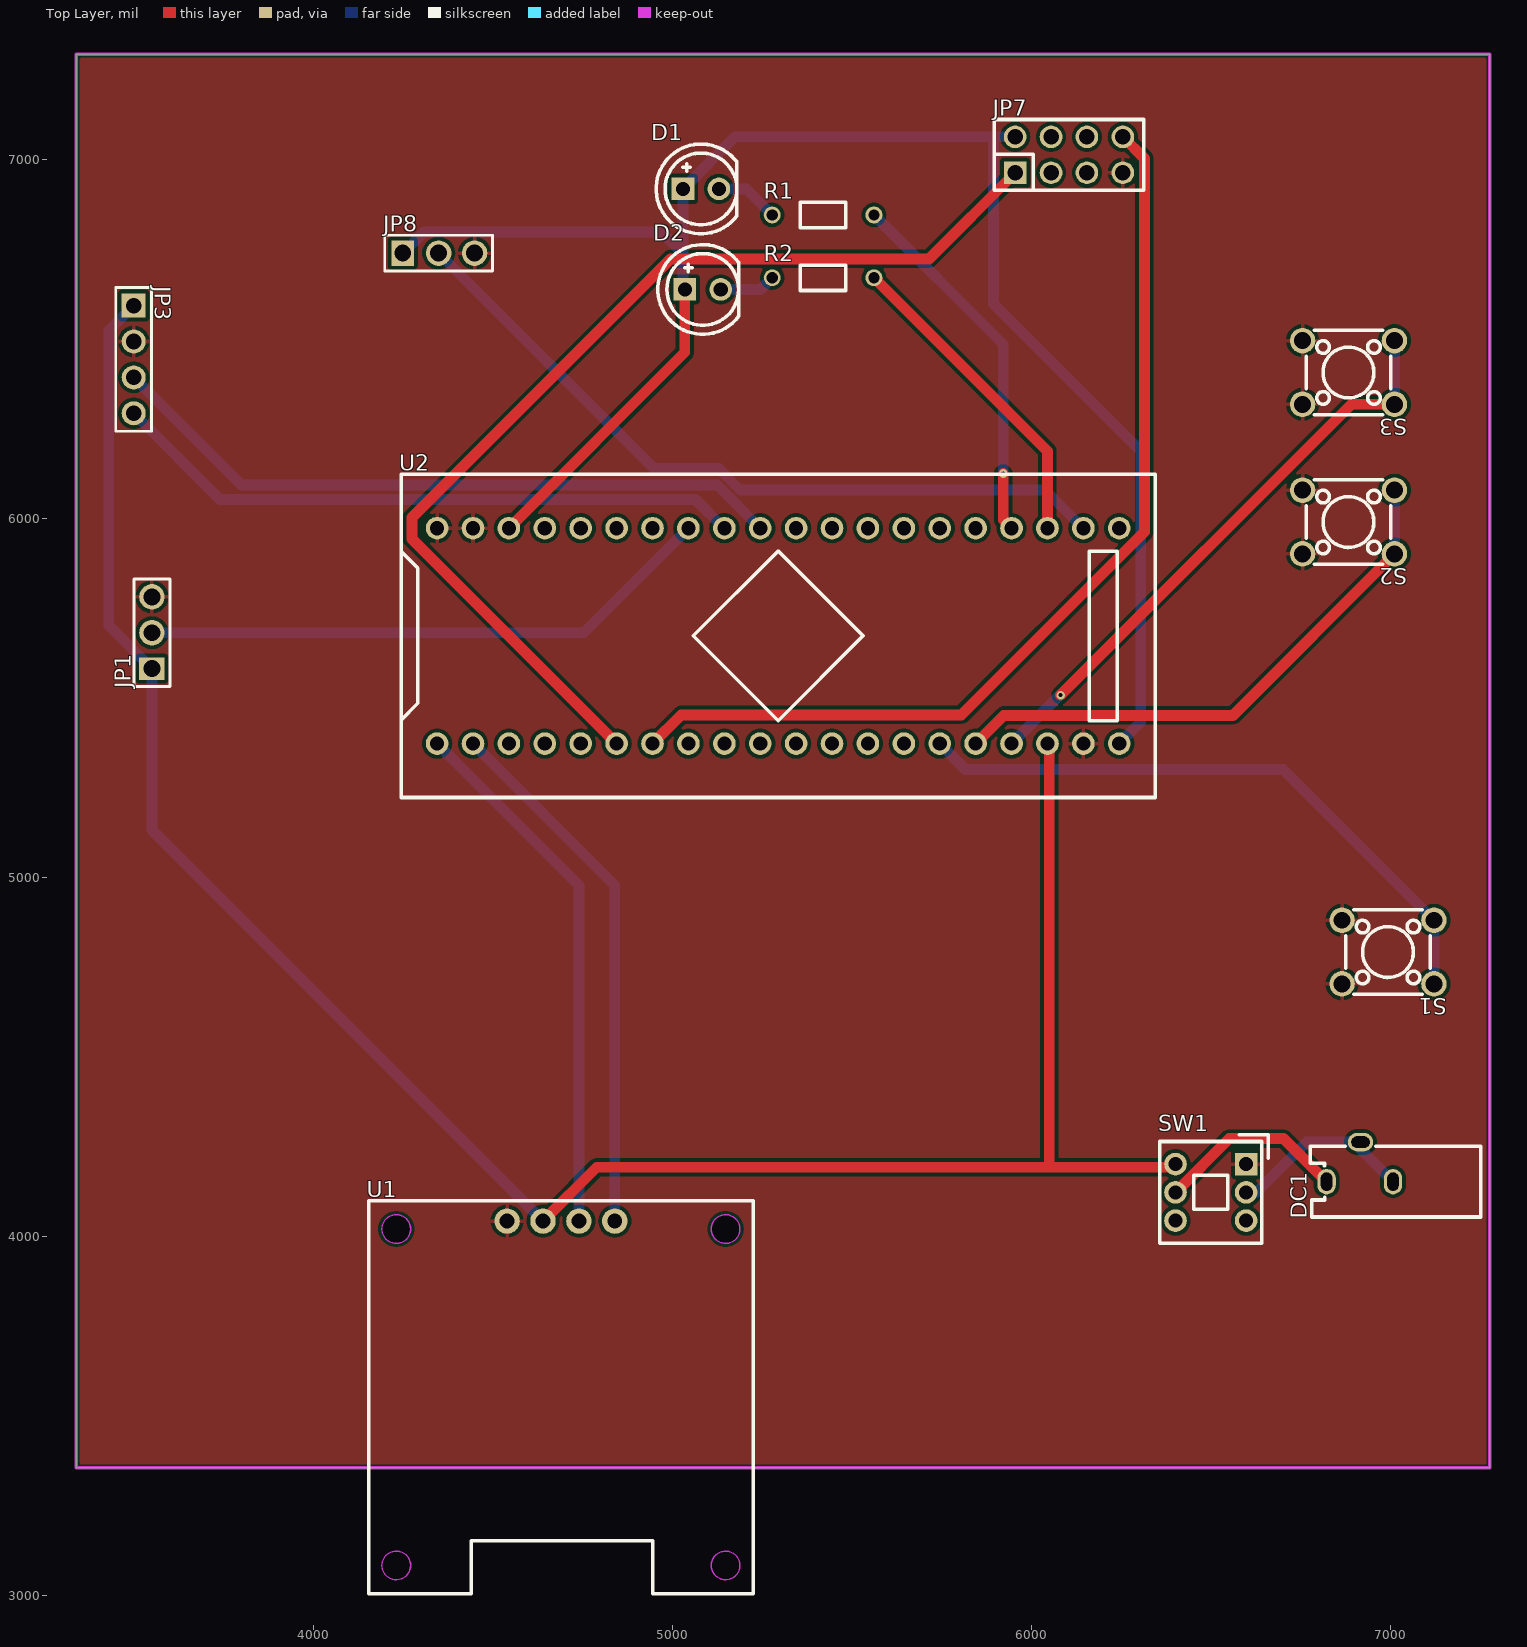
[diagram p0: Top Layer view]
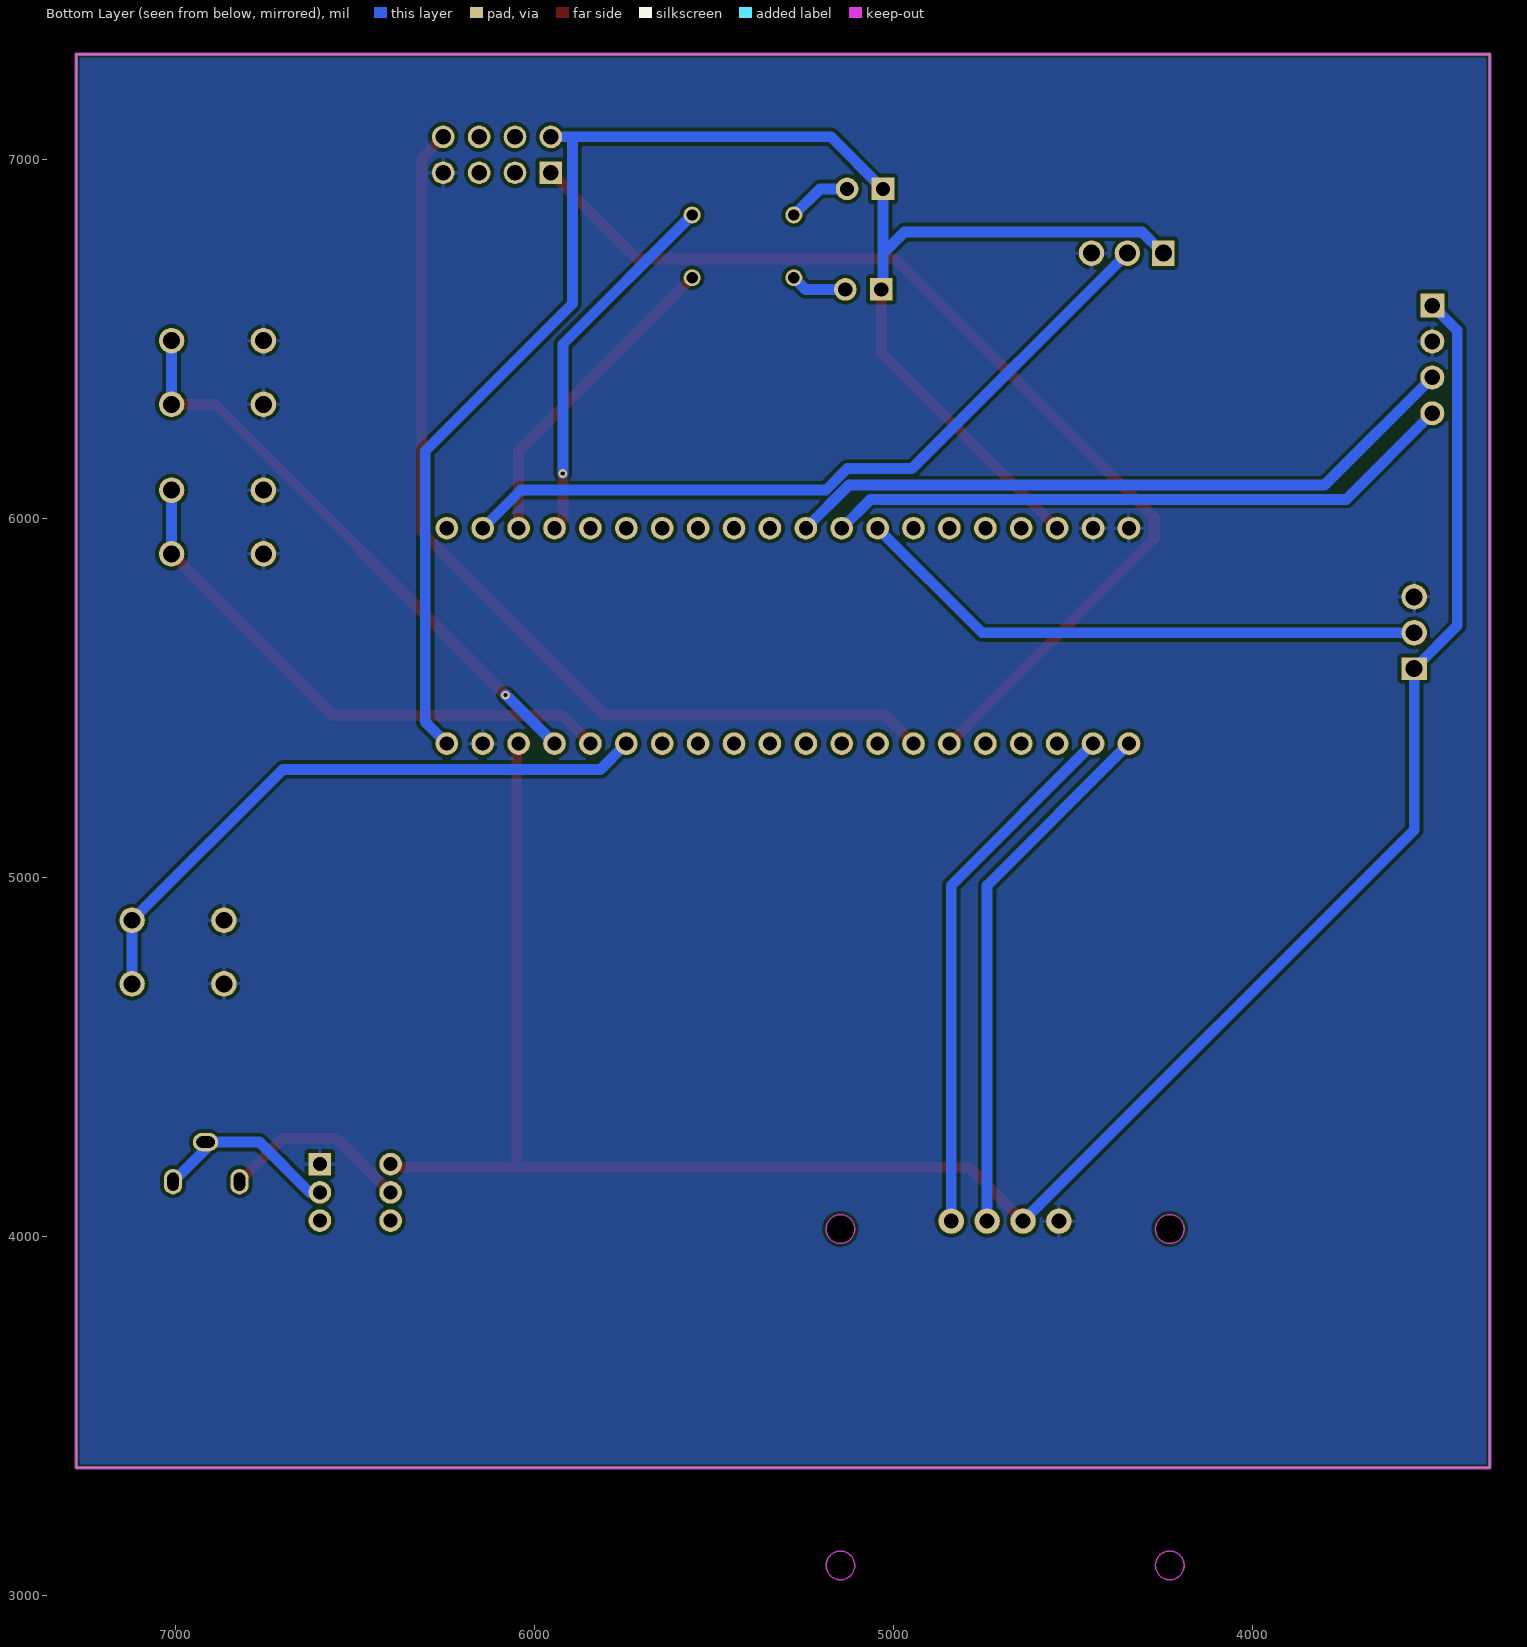
[diagram p1: Bottom Layer view, seen from below]
# Altium PCB MISC51894.pcbdoc
Units mil, origin at the board's own origin, x right, y up, seen from the top; angles counter-clockwise.
Board outline 3937.01 x 3937.01 mil, 2 copper layers (Top Layer, Bottom Layer), stack 62.206 mil thick; 15 components, 45 nets, 91 pads, 2 vias.

## Layer stack, top to bottom
Top Solder Mask Layer: solder mask 0.394, Dk 3.3
Top Layer: signal copper 1.379
Dielectric1: surface 59.449, FR4, Dk 4.5
Bottom Layer: signal copper 1.378
Bottom Solder Mask Layer: solder mask 0.394, Dk 3.3

## Board outline
3340,7292.79 3340,3355.79 7277.01,3355.79 7277.01,7292.79

## Design rules (kind name [scope] priority, off if disabled: settings)
BoardOutlineClearance copperThickness2oz_1 [All] p2 off: genericclearance=7.99 ignorepadtopadclearanceinfootprint=FALSE except(0: Arc-SplitContinuation Track-SplitContinuation SMDPad-SplitContinuation THPad-SplitContinuation Via-SplitContinuation Fill-SplitContinuation Region-SplitContinuation Poly-SplitContinuation Text-SplitContinuation Hole-SplitContinuation; 5.98: Arc-CutoutEdge SMDPad-CutoutEdge THPad-CutoutEdge Via-CutoutEdge Fill-CutoutEdge Region-CutoutEdge Text-CutoutEdge; 6.93: Hole-OutlineEdge Hole-CutoutEdge; 10: Poly-OutlineEdge Poly-CutoutEdge; 11.81: Arc-OutlineEdge Track-OutlineEdge SMDPad-OutlineEdge THPad-OutlineEdge Via-OutlineEdge Fill-OutlineEdge Region-OutlineEdge Text-OutlineEdge Track-CutoutEdge)
BoardOutlineClearance copperThickness1oz_1 [All] p4: genericclearance=4.02 ignorepadtopadclearanceinfootprint=FALSE except(0: Arc-SplitContinuation Track-SplitContinuation SMDPad-SplitContinuation THPad-SplitContinuation Via-SplitContinuation Fill-SplitContinuation Region-SplitContinuation Poly-SplitContinuation Text-SplitContinuation Hole-SplitContinuation; 6: SMDPad-CutoutEdge THPad-CutoutEdge Via-CutoutEdge Fill-CutoutEdge Region-CutoutEdge Text-CutoutEdge; 6.93: Hole-OutlineEdge Hole-CutoutEdge; 10: Poly-OutlineEdge Poly-CutoutEdge; 11.8: Arc-OutlineEdge Track-OutlineEdge SMDPad-OutlineEdge THPad-OutlineEdge Via-OutlineEdge Fill-OutlineEdge Region-OutlineEdge Text-OutlineEdge; 11.81: Arc-CutoutEdge Track-CutoutEdge)
Clearance copperThickness2oz [All] p1 off: gap=7.99 ignorepadtopadclearanceinfootprint=FALSE except(5.98: SMDPad-Track SMDPad-SMDPad THPad-Track SMDPad-THPad THPad-THPad Track-Via SMDPad-Via THPad-Via Via-Via Fill-Track Region-Track Fill-SMDPad Region-SMDPad Fill-THPad Region-THPad Fill-Via Region-Via Fill-Fill Fill-Region Region-Region Arc-Track Arc-SMDPad Arc-THPad Arc-Via Fill-Arc Region-Arc Arc-Arc Text-Track SMDPad-Text Text-THPad Text-Via Fill-Text Region-Text Arc-Text Text-Text; 6.93: Hole-Track Hole-SMDPad Hole-THPad Hole-Via Fill-Hole Region-Hole Hole-Arc Hole-Text; 10: Poly-Track Poly-SMDPad Poly-THPad Poly-Via Poly-Fill Poly-Region Poly-Poly Poly-Arc Poly-Text Poly-Hole)
Clearance copperThickness1oz [All] p3: gap=4.02 ignorepadtopadclearanceinfootprint=FALSE except(5.98: SMDPad-Track SMDPad-SMDPad THPad-Track SMDPad-THPad THPad-THPad Track-Via SMDPad-Via THPad-Via Via-Via Fill-Track Region-Track Fill-SMDPad Region-SMDPad Fill-THPad Region-THPad Fill-Via Region-Via Fill-Fill Fill-Region Region-Region; 6: Arc-Track Arc-SMDPad Arc-THPad Arc-Via Fill-Arc Region-Arc Arc-Arc Text-Track SMDPad-Text Text-THPad Text-Via Fill-Text Region-Text Arc-Text Text-Text; 6.93: Hole-Track Hole-SMDPad Hole-THPad Hole-Via Fill-Hole Region-Hole Hole-Arc Hole-Text; 10: Poly-Track Poly-SMDPad Poly-THPad Poly-Via Poly-Fill Poly-Region Poly-Poly Poly-Arc Poly-Text Poly-Hole)
Creepage creepage [All] p1: checkdistance=0 ignoreinternallayers=TRUE applytopolygonpour=TRUE
DiffPairsRouting differentialPair [All] p1: maxlimit=6 minlimit=6 mostfreqgap=6 toplayer_minwidth=5 toplayer_prefwidth=10 toplayer_maxwidth=100 toplayer_mingap=6 toplayer_prefgap=6 toplayer_maxgap=6 bottomlayer_minwidth=5 bottomlayer_prefwidth=10 bottomlayer_maxwidth=100 bottomlayer_mingap=6 bottomlayer_prefgap=6 bottomlayer_maxgap=6 maxuncoupledlength=10
HoleToHoleClearance otherClearance [All] p1: gap=11.81 allowstackedmicrovias=TRUE
Length netLength [All] p1: minlimit=0 maxlimit=0
MatchedLengths netLengthTolerance [All] p1: tolerance=1000
PasteMaskExpansion pasteMaskExpansion [All] p1: expansion=0
PlaneConnect innerPlane [All] p1: planeconnectstyle=Relief reliefexpansion=20 reliefentries=4 reliefconductorwidth=10 reliefairgap=10
PolygonConnect copperRegion [(InNet('GND'))] p1: connectstyle=Relief reliefconductorwidth=10 reliefentries=4 polygonreliefangle="90 Angle" airgapwidth=10 via.connectstyle=Relief via.reliefconductorwidth=10 via.reliefentries=4 via.polygonreliefangle="90 Angle" via.airgapwidth=10
RoutingVias viaSize [All] p1: holewidth=12.01 width=24.02 viastyle="Through Hole" minholewidth=11.81 minwidth=19.68 maxholewidth=248.03 maxwidth=393.7
SolderMaskExpansion solderMaskExpansion [IsVia] p1: expansion=-1000 istentingtop=TRUE
SolderMaskExpansion solderMaskExpansion [All] p2: expansion=2 istentingtop=FALSE
Width copperThickness2oz_2 [All] p1 off: maxlimit=100 minlimit=8 preferedwidth=10
Width copperThickness1oz_2 [All] p2: maxlimit=10 minlimit=10 preferedwidth=10 toplayer_minwidth=30 toplayer_maxwidth=100 toplayer_prefwidth=30 bottomlayer_minwidth=30 bottomlayer_maxwidth=100 bottomlayer_prefwidth=30

## Components (designator, comment, footprint, x,y, rotation, side; value= is the part's Value field where it differs from the comment)
D1 "led" LED-TH_5mm 5080,6917.79 r0 top
D2 "led" LED-TH_5mm 5085,6637.79 r0 top
DC1 "DC002-1.3" DC-IN-TH_DC002-1.3 6915,4207.79 r90 top
JP1 "HDR-1X3" HDR-TH_3P-P2.54-V-M-1 3550.66,5681.57 r90 top
JP3 "HDR-1X4" HDR-TH_4P-P2.54-V-M-1 3500,6442.79 r270 top
JP7 "Header 4X2" HDR-TH_8P-P2.54-V-F-R2-C4-S2.54-1 6105,7012.79 r0 top
JP8 "HDR-1X3" HDR-TH_3P-P2.54-V-M-1 4349.37,6738.79 r0 top
R1 "Res2" Res_1/8W 5420,6842.79 r0 top
R2 "Res2" Res_1/8W 5420,6667.79 r0 top
S1 "key_4" SW-TH_4P-L6.0-W6.0-P4.50-LS6.5 6993.59,4792.23 r180 top
S2 "key_4" SW-TH_4P-L6.0-W6.0-P4.50-LS6.5 6883.59,5989.94 r180 top
S3 "key_4" SW-TH_4P-L6.0-W6.0-P4.50-LS6.5 6883.59,6406.5 r180 top
SW1 "Self-lock button" SW-TH_6P-L7.0-W7.0-P2.00 6500,4122.79 r0 top
U1 "OLED" OLED-TH_L27.8-W27.2-P2.54_C9900033791 4690,4042.79 r0 top
U2 "STM32F103C8T6-Card" CONN-TH_L53.3-W22.9_STM32F103C8T6-CARD 5295,5672.79 r0 top

## Footprints (in the part's own frame and the unit in brackets; to place one, negate y for a bottom-side part, rotate by r counter-clockwise, add the part's x,y. Pads: shape width x height; smd on the part's side, far side on the other; paste and mask are expansions set on the pad)
CONN-TH_L53.3-W22.9_STM32F103C8T6-CARD [mm]
  round 1.6 hole 1: 1(-24.13,-7.62) 2(-21.59,-7.62) 3(-19.05,-7.62) 4(-16.51,-7.62) 5(-13.97,-7.62) 6(-11.43,-7.62) 7(-8.89,-7.62) 8(-6.35,-7.62) 9(-3.81,-7.62) 10(-1.27,-7.62) 11(1.27,-7.62) 12(3.81,-7.62) 13(6.35,-7.62) 14(8.89,-7.62) 15(11.43,-7.62) 16(13.97,-7.62) 17(16.51,-7.62) 18(19.05,-7.62) 19(21.59,-7.62) 20(24.13,-7.62) 21(24.13,7.62) 22(21.59,7.62) 23(19.05,7.62) 24(16.51,7.62) 25(13.97,7.62) 26(11.43,7.62) 27(8.89,7.62) 28(6.35,7.62) 29(3.81,7.62) 30(1.27,7.62) 31(-1.27,7.62) 32(-3.81,7.62) 33(-6.35,7.62) 34(-8.89,7.62) 35(-11.43,7.62) 36(-13.97,7.62) 37(-16.51,7.62) 38(-19.05,7.62) 39(-21.59,7.62) 40(-24.13,7.62)
  silkscreen extent -26.67,-11.43 26.67,11.43
DC-IN-TH_DC002-1.3 [mm]
  oval 1.8x1.3 hole 0.8 slot 1.3 at 0 deg paste+0 mask+0.05: 1(-1.4,2.35) 3(-1.4,-2.35)
  oval 1.3x1.8 hole 0.8 slot 1.3 at 90 deg paste+0 mask+0.05: 2(1.4,-0.05)
  silkscreen extent -3.9,-8.55 1.1,3.5
HDR-TH_3P-P2.54-V-M-1 [mm]
  rect 1.575x1.8 hole 1.2: 1(-2.54,0)
  round 1.8 hole 1.2: 2(0,0) 3(2.54,0)
  silkscreen extent -3.81,-1.27 3.81,1.27
HDR-TH_4P-P2.54-V-M-1 [mm]
  rect 1.7x1.7 hole 1.1: 1(-3.81,0)
  round 1.7 hole 1.1: 2(-1.27,0) 3(1.27,0) 4(3.81,0)
  silkscreen extent -5.08,-1.27 5.08,1.27
HDR-TH_8P-P2.54-V-F-R2-C4-S2.54-1 [mm]
  rect 1.6x1.6 hole 1.1: 1(-3.81,-1.27)
  round 1.6 hole 1.1: 2(-3.81,1.27) 3(-1.27,-1.27) 4(-1.27,1.27) 5(1.27,-1.27) 6(1.27,1.27) 7(3.81,-1.27) 8(3.81,1.27)
  silkscreen extent -5.28,-2.5 5.28,2.5
LED-TH_5mm [mm]
  rect 1.6x1.6 hole 1 paste+0 mask+0.051: 1(-1.27,0)
  round 1.6 hole 1 paste+0 mask+0.051: 2(1.27,0)
  silkscreen extent -3.17,-3.17 2.54,3.17
OLED-TH_L27.8-W27.2-P2.54_C9900033791 [mm]
  round 1.8 hole 1.05 paste+0 mask+0.05: 1(-3.81,0) 2(-1.27,0) 3(1.27,0) 4(3.81,0)
  Board Outline Layer circle w0.003: c-11.65,-0.56 r1.016
  Board Outline Layer circle w0.003: c11.65,-0.56 r1.016
  Board Outline Layer circle w0.003: c-11.65,-24.36 r1.016
  Board Outline Layer circle w0.003: c11.65,-24.36 r1.016
  Board Outline Layer region: -10.634,-0.56 -10.735,-1.001 -11.016,-1.354 -11.424,-1.551 -11.876,-1.551 -12.283,-1.354 -12.565,-1.001 -12.666,-0.56 -12.666,-0.56 -12.565,-0.119 -12.283,0.234 -11.876,0.431 -11.424,0.431 -11.016,0.234 -10.735,-0.119 -10.634,-0.56
  Board Outline Layer region: -10.634,-0.56 -10.643,-0.698 -10.672,-0.834 -10.718,-0.965 -10.782,-1.088 -10.862,-1.201 -10.956,-1.303 -11.064,-1.39 -11.183,-1.462 -11.31,-1.517 -11.443,-1.555 -11.581,-1.574 -11.719,-1.574 -11.857,-1.555 -11.99,-1.517 -12.117,-1.462 -12.236,-1.39 -12.343,-1.303 -12.438,-1.201 -12.518,-1.088 -12.582,-0.965 -12.628,-0.834 -12.656,-0.698 -12.666,-0.56 -12.656,-0.422 -12.628,-0.286 -12.582,-0.155 -12.518,-0.032 -12.438,0.081 -12.343,0.183 -12.236,0.27 -12.117,0.342 -11.99,0.397 -11.857,0.435 -11.719,0.454 -11.581,0.454 -11.443,0.435 -11.31,0.397 -11.183,0.342 -11.064,0.27 -10.956,0.183 -10.862,0.081 -10.782,-0.032 -10.718,-0.155 -10.672,-0.286 -10.643,-0.422
  Board Outline Layer region: 12.666,-0.56 12.565,-1.001 12.283,-1.354 11.876,-1.551 11.424,-1.551 11.017,-1.354 10.735,-1.001 10.634,-0.56 10.634,-0.56 10.735,-0.119 11.017,0.234 11.424,0.431 11.876,0.431 12.283,0.234 12.565,-0.119 12.666,-0.56
  Board Outline Layer region: 12.666,-0.56 12.657,-0.698 12.628,-0.834 12.582,-0.965 12.518,-1.088 12.438,-1.201 12.343,-1.303 12.236,-1.39 12.117,-1.462 11.99,-1.517 11.857,-1.555 11.719,-1.574 11.581,-1.574 11.443,-1.555 11.31,-1.517 11.183,-1.462 11.064,-1.39 10.957,-1.303 10.862,-1.201 10.782,-1.088 10.718,-0.965 10.672,-0.834 10.643,-0.698 10.634,-0.56 10.643,-0.422 10.672,-0.286 10.718,-0.155 10.782,-0.032 10.862,0.081 10.957,0.183 11.064,0.27 11.183,0.342 11.31,0.397 11.443,0.435 11.581,0.454 11.719,0.454 11.857,0.435 11.99,0.397 12.117,0.342 12.236,0.27 12.343,0.183 12.438,0.081 12.518,-0.032 12.582,-0.155 12.628,-0.286 12.657,-0.422
  Board Outline Layer region: -10.634,-24.36 -10.735,-24.801 -11.016,-25.154 -11.424,-25.35 -11.876,-25.35 -12.283,-25.154 -12.565,-24.801 -12.666,-24.36 -12.666,-24.36 -12.565,-23.919 -12.283,-23.566 -11.876,-23.369 -11.424,-23.369 -11.016,-23.566 -10.735,-23.919 -10.634,-24.36
  Board Outline Layer region: -10.634,-24.36 -10.643,-24.498 -10.672,-24.634 -10.718,-24.765 -10.782,-24.888 -10.862,-25.001 -10.956,-25.102 -11.064,-25.19 -11.183,-25.262 -11.31,-25.317 -11.443,-25.355 -11.581,-25.374 -11.719,-25.374 -11.857,-25.355 -11.99,-25.317 -12.117,-25.262 -12.236,-25.19 -12.343,-25.102 -12.438,-25.001 -12.518,-24.888 -12.582,-24.765 -12.628,-24.634 -12.656,-24.498 -12.666,-24.36 -12.656,-24.222 -12.628,-24.086 -12.582,-23.955 -12.518,-23.832 -12.438,-23.719 -12.343,-23.617 -12.236,-23.53 -12.117,-23.458 -11.99,-23.403 -11.857,-23.365 -11.719,-23.346 -11.581,-23.346 -11.443,-23.365 -11.31,-23.403 -11.183,-23.458 -11.064,-23.53 -10.956,-23.617 -10.862,-23.719 -10.782,-23.832 -10.718,-23.955 -10.672,-24.086 -10.643,-24.222
  Board Outline Layer region: 12.666,-24.36 12.565,-24.801 12.283,-25.154 11.876,-25.35 11.424,-25.35 11.017,-25.154 10.735,-24.801 10.634,-24.36 10.634,-24.36 10.735,-23.919 11.017,-23.566 11.424,-23.369 11.876,-23.369 12.283,-23.566 12.565,-23.919 12.666,-24.36
  Board Outline Layer region: 12.666,-24.36 12.657,-24.498 12.628,-24.634 12.582,-24.765 12.518,-24.888 12.438,-25.001 12.343,-25.102 12.236,-25.19 12.117,-25.262 11.99,-25.317 11.857,-25.355 11.719,-25.374 11.581,-25.374 11.443,-25.355 11.31,-25.317 11.183,-25.262 11.064,-25.19 10.957,-25.102 10.862,-25.001 10.782,-24.888 10.718,-24.765 10.672,-24.634 10.643,-24.498 10.634,-24.36 10.643,-24.222 10.672,-24.086 10.718,-23.955 10.782,-23.832 10.862,-23.719 10.957,-23.617 11.064,-23.53 11.183,-23.458 11.31,-23.403 11.443,-23.365 11.581,-23.346 11.719,-23.346 11.857,-23.365 11.99,-23.403 12.117,-23.458 12.236,-23.53 12.343,-23.617 12.438,-23.719 12.518,-23.832 12.582,-23.955 12.628,-24.086 12.657,-24.222
  Multi-Layer board cut-out: -10.634,-0.56 -10.735,-1.001 -11.016,-1.354 -11.424,-1.551 -11.876,-1.551 -12.283,-1.354 -12.565,-1.001 -12.666,-0.56 -12.666,-0.56 -12.565,-0.119 -12.283,0.234 -11.876,0.431 -11.424,0.431 -11.016,0.234 -10.735,-0.119 -10.634,-0.56
  Multi-Layer board cut-out: 12.666,-0.56 12.565,-1.001 12.283,-1.354 11.876,-1.551 11.424,-1.551 11.017,-1.354 10.735,-1.001 10.634,-0.56 10.634,-0.56 10.735,-0.119 11.017,0.234 11.424,0.431 11.876,0.431 12.283,0.234 12.565,-0.119 12.666,-0.56
  Multi-Layer board cut-out: -10.634,-24.36 -10.735,-24.801 -11.016,-25.154 -11.424,-25.35 -11.876,-25.35 -12.283,-25.154 -12.565,-24.801 -12.666,-24.36 -12.666,-24.36 -12.565,-23.919 -12.283,-23.566 -11.876,-23.369 -11.424,-23.369 -11.016,-23.566 -10.735,-23.919 -10.634,-24.36
  Multi-Layer board cut-out: 12.666,-24.36 12.565,-24.801 12.283,-25.154 11.876,-25.35 11.424,-25.35 11.017,-25.154 10.735,-24.801 10.634,-24.36 10.634,-24.36 10.735,-23.919 11.017,-23.566 11.424,-23.369 11.876,-23.369 12.283,-23.566 12.565,-23.919 12.666,-24.36
  silkscreen extent -13.6,-26.36 13.6,1.44
Res_1/8W [mil]
  round 47.2 hole 31.5 paste+0 mask+2: 1(-141.7,2.48) 2(141.7,2.48)
  silkscreen extent -63,-33 63,38
SW-TH_4P-L6.0-W6.0-P4.50-LS6.5 [mm]
  round 1.8 hole 1.2: 1(-3.25,2.25) 2(3.25,2.25) 3(-3.25,-2.25) 4(3.25,-2.25)
  silkscreen extent -3,-3 3,3
SW-TH_6P-L7.0-W7.0-P2.00 [mm]
  rect 1.6x1.6 hole 1: 1(2.5,2)
  round 1.6 hole 1: 2(2.5,0) 3(2.5,-2) 4(-2.5,2) 5(-2.5,0) 6(-2.5,-2)
  silkscreen extent -3.6,-3.6 4.06,4.06

## Via types
v1: diameter 24.02, hole 12, Top Layer to Bottom Layer, 2 vias

## Nets (pads, with @x,y where several pads share a name; then routed paths per layer and width w, separated by ;. In a path a pad name is that pad's centre, name@x,y a point inside that pad or via, vN(x,y) a via of type N, cw(c..) or ccw(c..) an arc to the next point about the centre after c; other vN are vias at no path point)
$2N1: D1.2 R1.1 | length 178.3
  Bottom Layer w30: D1.2 5205.78,6917.79 R1.1
$2N5: D2.2 R2.1 | length 156.8
  Bottom Layer w30: D2.2 5245.82,6637.79 R2.1
$2N24: JP7.3
$2N25: JP7.5
$2N28: JP7.4
$2N29: JP7.6
$2N54: U2.37
$2N70: U2.21
+3: D1.1 D2.1 JP7.2 JP8.1 U2.20 U2.38 | length 4849.7
  Top Layer w30: U2.38 5035,6462.79 D2.1
  Bottom Layer w30: JP8.1 4308.37,6797.79 4970,6797.79 5030,6737.79 ; D2.1 5030,6642.79 5030,6737.79 ; JP7.2 5895,7062.79 ; U2.20 6305,5432.79 6305,6187.83 5895,6597.83 5895,7062.79 ; 5030,6737.79 D1.1 5175,7062.79 5895,7062.79
+5: JP1.1 JP3.1 SW1.4 U1.2 U2.18 | length 6089
  Top Layer w30: U1.2 4790,4192.79 6050,4192.79 ; U2.18 6050,5367.8 6050,4192.79 ; SW1.4 6392.83,4192.79 6050,4192.79
  Bottom Layer w30: JP3.1 3430.66,6523.45 3430.66,5701.57 JP1.1 3550.66,5132.13 U1.2
DC_GND: DC1.2 DC1.3 SW1.2 | length 524.3
  Bottom Layer w30: SW1.2 6626.85,4122.79 6766.97,4262.91 DC1.2 6916.97,4243.23 DC1.3
DC_VCC: DC1.1 SW1.5 | length 532.7
  Top Layer w30: SW1.5 6551.46,4272.68 6702.48,4272.68 DC1.1
GND: JP1.3 JP3.2 JP7.7 JP8.3 S1.2 S1.4 S2.2 S2.4 S3.2 S3.4 SW1.1 U1.1 U2.19 U2.39 U2.40
PA0: U2.25
PA1: U2.26
PA2: U2.27
PA3: U2.28
PA4: U2.29
PA5: U2.30
PA6: JP3.3 U2.31 | length 1919
  Bottom Layer w30: JP3.3 3800,6092.8 5125,6092.8 U2.31
PA7: JP3.4 U2.32 | length 1777.6
  Bottom Layer w30: JP3.4 3740,6052.8 5065,6052.8 U2.32
PA8: U2.5
PA9: JP7.1 U2.6 | length 2943.7
  Top Layer w30: U2.6 4275,5942.79 4275,6002.8 4995,6722.79 5715,6722.79 JP7.1
PA10: JP7.8 U2.7 | length 2739.2
  Top Layer w30: U2.7 5025,5452.79 5805,5452.79 6315,5962.79 6315,7002.79 JP7.8
PA11: U2.8
PA12: U2.9
PA15: U2.10
PB0: JP1.2 U2.33 | length 1615
  Bottom Layer w30: JP1.2 4753.78,5681.57 U2.33
PB1: U2.34
PB3: U2.11
PB4: U2.12
PB5: U2.13
PB6: U2.14
PB7: S1.1 S1.3 U2.15 | length 1757.5
  Bottom Layer w30: U2.15 5816.99,5300.81 6701.54,5300.81 S1.3 S1.1@7121.54,4703.65
PB8: S2.1 S2.3 U2.16 | length 1562.6
  Top Layer w30: U2.16 5923.58,5451.36 6561.54,5451.36 S2.1
  Bottom Layer w30: S2.1 S2.3
PB9: S3.1 S3.3 U2.17 | length 1635.2
  Top Layer w30: v1(6081.54,5507.93) 6891.54,6317.92 S3.1
  Bottom Layer w30: U2.17 6080.14,5507.93 v1(6081.54,5507.93) ; S3.1 S3.3
PB10: U2.35
PB11: U2.36
PB12: U1.3 U2.1 | length 1493.6
  Bottom Layer w30: U2.1 4740,4977.8 U1.3
PB13: U1.4 U2.2 | length 1493.6
  Bottom Layer w30: U2.2 4840,4977.8 U1.4
PB14: U2.3
PB15: U2.4
PC13: JP8.2 U2.22 | length 2112.9
  Bottom Layer w30: JP8.2 4949.37,6138.8 5129.37,6138.8 5189.37,6078.8 6039,6078.8 U2.22
PC14: R2.2 U2.23 | length 897.7
  Top Layer w30: R2.2 6045,6186.97 U2.23
PC15: R1.2 U2.24 | length 1031.2
  Top Layer w30: v1(5921.7,6125.27) 5921.7,5996.09 U2.24
  Bottom Layer w30: R1.2 5921.7,6485.27 v1(5921.7,6125.27)
pads on no net: SW1.3 SW1.6

## Polygon pours and split planes (outlines as drawn)
GND on Top Layer (solid, remove dead copper, pour order 0): 3000,7472.79 3000,3112.79 7845,3112.79 7845,7472.79
GND on Bottom Layer (solid, remove dead copper, pour order 2): 3085,7392.79 3085,3162.79 7715,3162.79 7715,7392.79

## Keep-outs
Board Outline Layer:
  the board outline again, w10